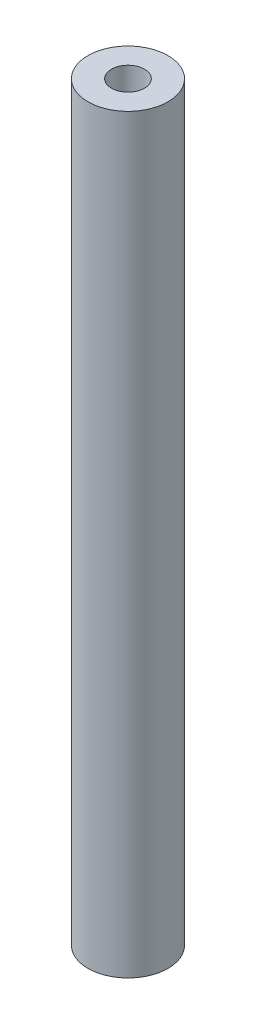
from build123d import *

# Parameters (mm, degrees)
SKETCH_1_R             = 4
EXTRUDE_1_DEPTH        = 75
HOLE_WIZARD_M4_1_D     = 3.3
HOLE_WIZARD_M4_1_DEPTH = 10.1
HOLE_WIZARD_M4_1_TIP   = 0.991420021


with BuildPart() as part:
    # 草图1 → 凸台-拉伸1 (new body)
    with BuildSketch(Plane(origin=(0, 0, 0), x_dir=(1, 0, 0), z_dir=(0, 1, 0))):
        with Locations(Location((0, 0, 0), (0, 0, 270))):
            Circle(SKETCH_1_R)
    extrude(amount=EXTRUDE_1_DEPTH)

    # M4 螺纹孔1
    with Locations(Plane(origin=(0, 75, 0), x_dir=(1, 0, 0), z_dir=(0, 1, 0))):
        with Locations((0, 0)):
            Hole(HOLE_WIZARD_M4_1_D / 2, depth=HOLE_WIZARD_M4_1_DEPTH)
            with Locations((0, 0, -(HOLE_WIZARD_M4_1_DEPTH + HOLE_WIZARD_M4_1_TIP / 2))):  # 118° drill point
                Cone(0, HOLE_WIZARD_M4_1_D / 2, HOLE_WIZARD_M4_1_TIP, mode=Mode.SUBTRACT)


solid = part.part
